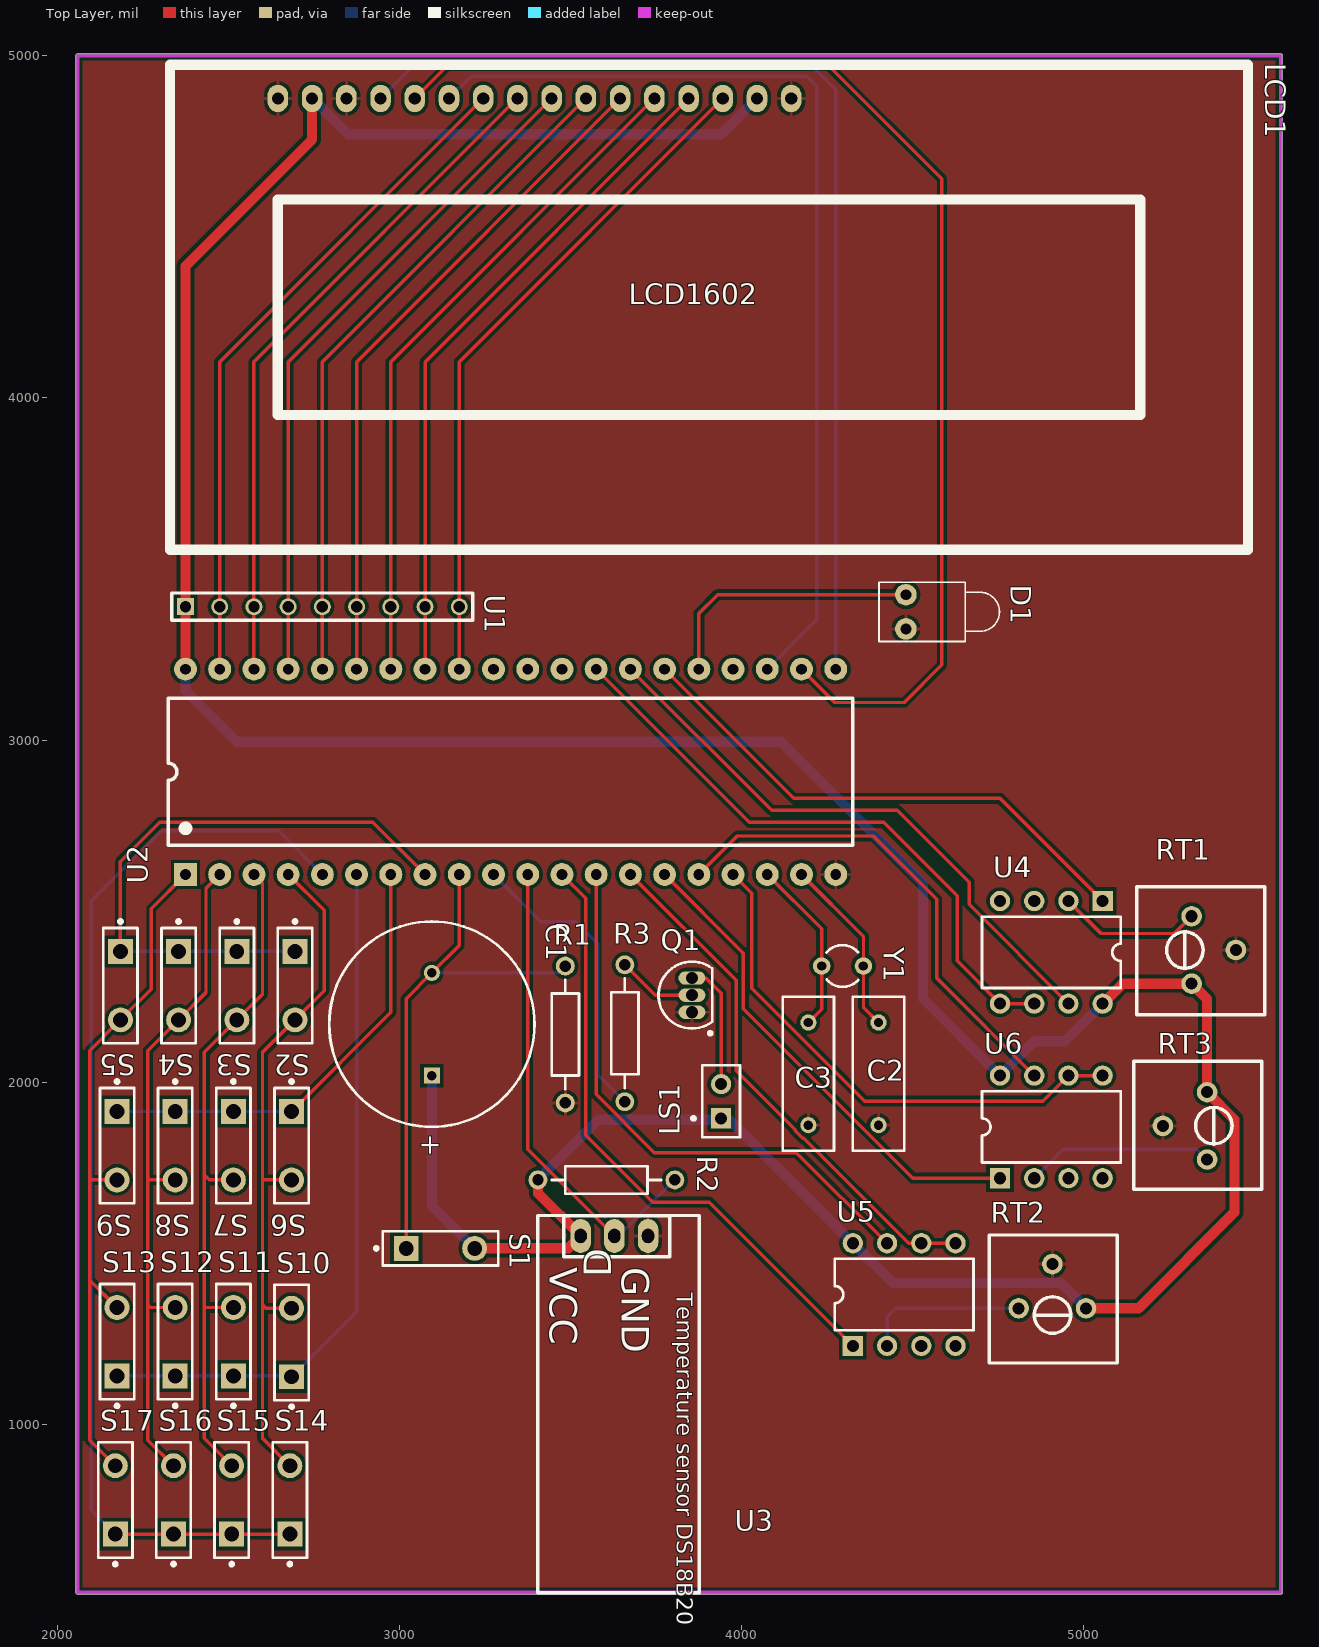
[diagram p0: Top Layer view]
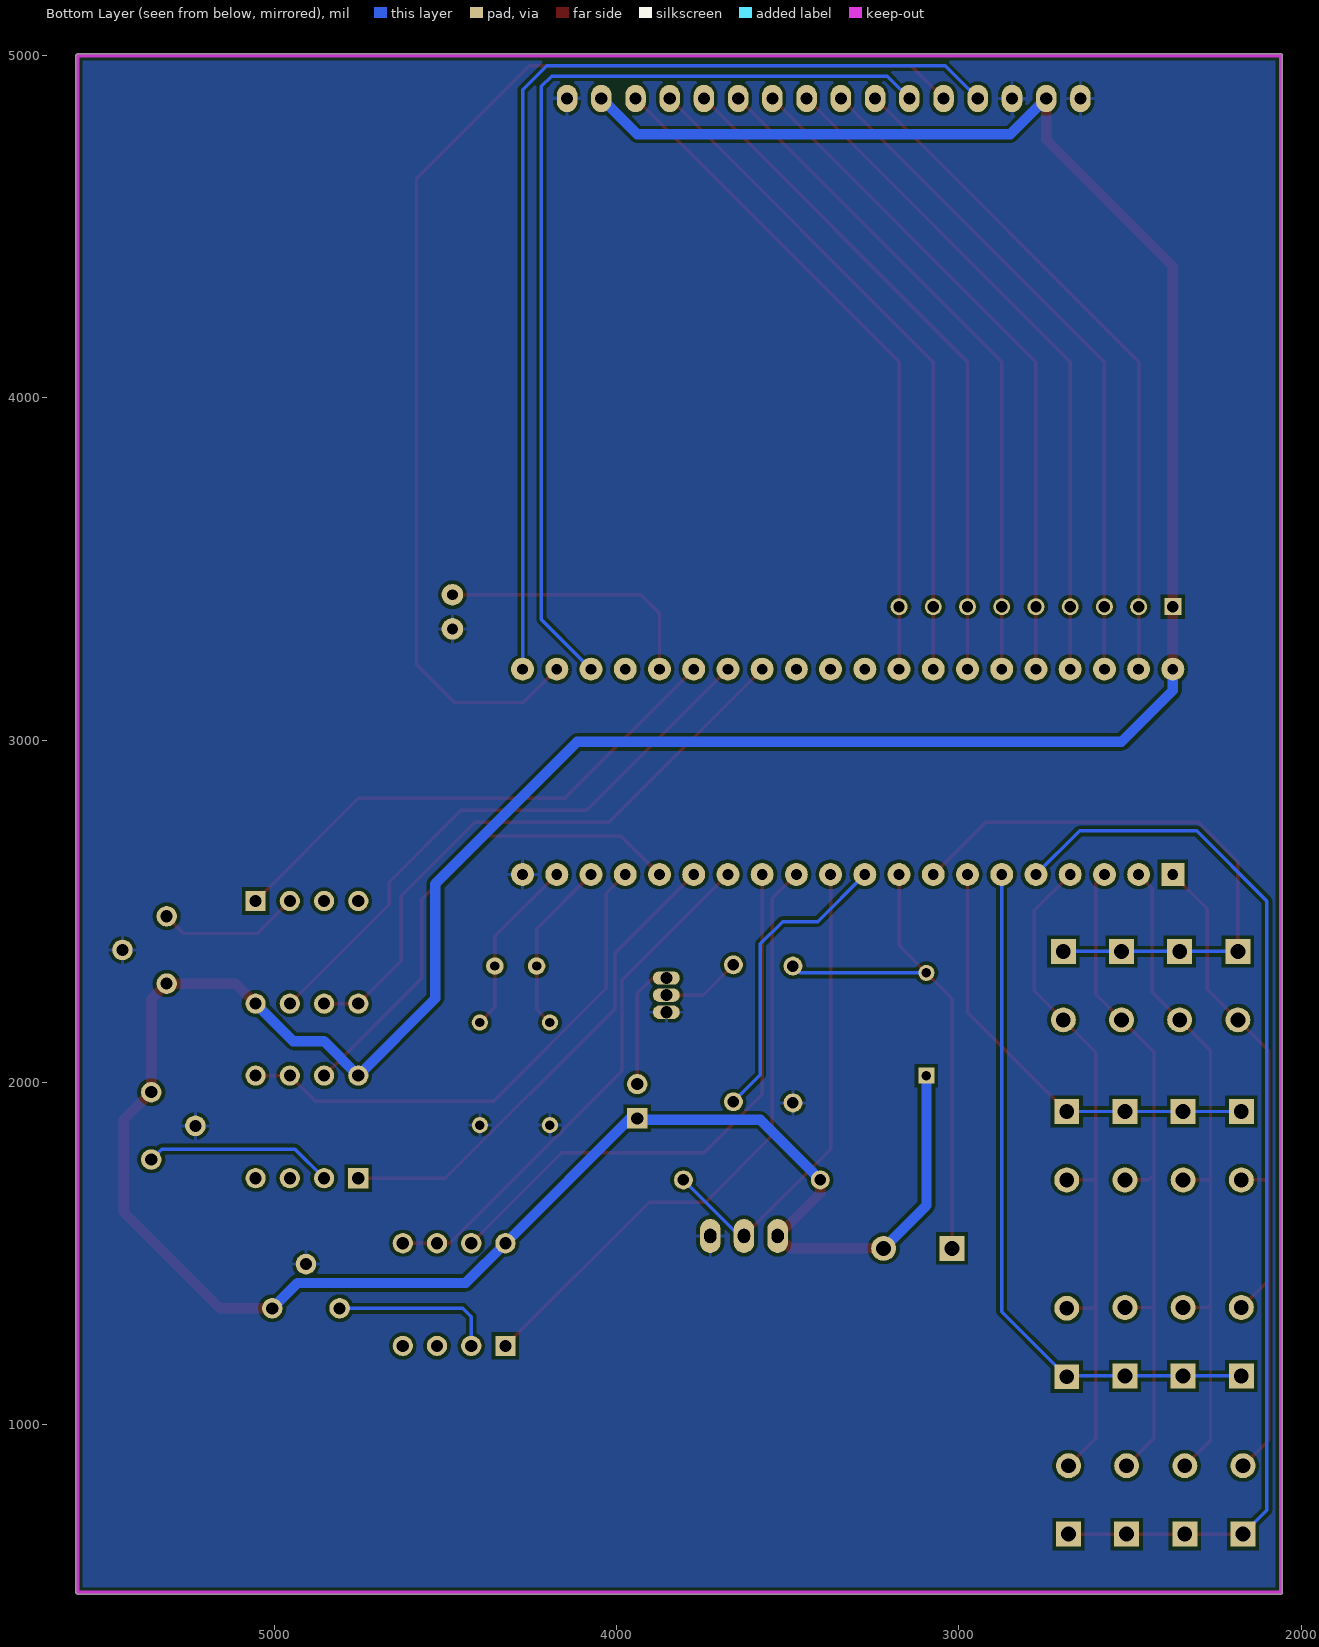
[diagram p1: Bottom Layer view, seen from below]
# Altium PCB MISC80677.PcbDoc
Units mil, origin at the board's own origin, x right, y up, seen from the top; angles counter-clockwise.
Board outline 3525.03 x 4500.03 mil, 2 copper layers (Top Layer, Bottom Layer); 37 components, 42 nets, 156 pads, 0 vias.

## Layer stack, top to bottom (the 12.6 mil dielectric is the usual default, probably not edited)
Top Solder: solder mask 0.4, Solder Resist, Dk 3.5
Top Layer: signal copper 1.4
Dielectric 1: dielectric 12.6, FR-4, Dk 4.8
Bottom Layer: signal copper 1.4
Bottom Solder: solder mask 0.4, Solder Resist, Dk 3.5

## Board outline
2054.99,510 ccw(c2060,510) 2060,504.99 5575,504.99 ccw(c5575,510) 5580.02,510 5580.02,5000 ccw(c5575,5000) 5575,5005.02 2060,5005.02 ccw(c2060,5000) 2054.99,5000

## Design rules (kind name [scope] priority, off if disabled: settings)
Clearance [All] p1: gap=10
MinimumSolderMaskSliver [All] p1: minsoldermaskwidth=0
PolygonConnect [All] p1: connectstyle=Relief reliefconductorwidth=10 reliefentries=4 polygonreliefangle="90 Angle" airgapwidth=10
RoutingVias [All] p1: holewidth=28 width=50 viastyle="Through Hole" minholewidth=28 minwidth=50 maxholewidth=28 maxwidth=50
SilkToSilkClearance [All] p1: silktosilkclearance=0
SilkToSolderMaskClearance [IsPad] p1: minsilkscreentomaskgap=0 clearancetoexposedcopper=TRUE
SolderMaskExpansion [All] p1: expansion=4
Width [All] p1: maxlimit=30 minlimit=10 preferedwidth=10
27 further rules are at their usual default settings.

## Components (designator, comment, footprint, x,y, rotation, side; value= is the part's Value field where it differs from the comment)
C1 "1UF" RB7.6-15 3095,2170 r270 top
C2 "22PF" RAD-0.3 4400,2025 r90 top
C3 "22PF" RAD-0.3 4195,2025 r90 top
D1 "LED1" LED-1 4480,3375 r0 top
LCD1 "LCD1602" LCD1602 2645,4875 r0 top
LS1 "Speaker" PIN2 3940,1895 r90 top
Q1 "2N3904" TO-92A 3855,2255 r0 top
R1 "1K" AXIAL-0.4 3485,2140 r90 top
R2 "1K" AXIAL-0.4 3605,1715 r0 top
R3 "1K" AXIAL-0.4 3658.94,2143.44 r90 top
RT1 "1K" 电位器 5330,2385 r270 top
RT2 "1K" 电位器 4910,1355 r0 top
RT3 "1K" 电位器 5345,1875 r90 top
S1 "SW-PB" SPST-2 3120,1515 r0 top
S2 "SW-PB" SPST-2 2695,2282.72 r270 top
S3 "SW-PB" SPST-2 2525,2282.72 r270 top
S4 "SW-PB" SPST-2 2355,2282.72 r270 top
S5 "SW-PB" SPST-2 2185,2282.72 r270 top
S6 "SW-PB" SPST-2 2685,1815 r270 top
S7 "SW-PB" SPST-2 2515,1815 r270 top
S8 "SW-PB" SPST-2 2345,1815 r270 top
S9 "SW-PB" SPST-2 2175,1815 r270 top
S10 "SW-PB" SPST-2 2685,1240 r90 top
S11 "SW-PB" SPST-2 2515,1242.28 r90 top
S12 "SW-PB" SPST-2 2345,1242.28 r90 top
S13 "SW-PB" SPST-2 2175,1242.28 r90 top
S14 "SW-PB" SPST-2 2680,780 r90 top
S15 "SW-PB" SPST-2 2510,780 r90 top
S16 "SW-PB" SPST-2 2340,780 r90 top
S17 "SW-PB" SPST-2 2170,780 r90 top
U1 "Resistor network" paizu 2775,3390 r0 top
U2 "AT89C52" DIP40 3325,2907.46 r90 top
U3 "DS18B20" DS18B20 3640,1060 r270 top
U4 "ADC0832CCN" N08E 4905,2380 r180 top
U5 "ADC0832CCN" N08E 4475,1380 r0 top
U6 "ADC0832CCN" N08E 4905,1870 r0 top
Y1 "12MHZ" R38 4295,2340 r270 top

## Footprints (in the part's own frame and the unit in brackets; to place one, negate y for a bottom-side part, rotate by r counter-clockwise, add the part's x,y. Pads: shape width x height; smd on the part's side, far side on the other; paste and mask are expansions set on the pad)
AXIAL-0.4 [mm] "Axial Device, Thru-Hole; 2 Leads; 0.4 in Pin Spacing"
  round 1.4 hole 0.85: 1(-5.08,0) 2(5.08,0)
  silkscreen extent -4.06,-1.02 4.06,1.02
DIP40 [mm]
  rect 1.7x1.7 hole 0.8: 1(-7.62,24.13)
  round 1.7 hole 0.8: 2(-7.62,21.59) 3(-7.62,19.05) 4(-7.62,16.51) 5(-7.62,13.97) 6(-7.62,11.43) 7(-7.62,8.89) 8(-7.62,6.35) 9(-7.62,3.81) 10(-7.62,1.27) 11(-7.62,-1.27) 12(-7.62,-3.81) 13(-7.62,-6.35) 14(-7.62,-8.89) 15(-7.62,-11.43) 16(-7.62,-13.97) 17(-7.62,-16.51) 18(-7.62,-19.05) 19(-7.62,-21.59) 20(-7.62,-24.13) 21(7.62,-24.13) 22(7.62,-21.59) 23(7.62,-19.05) 24(7.62,-16.51) 25(7.62,-13.97) 26(7.62,-11.43) 27(7.62,-8.89) 28(7.62,-6.35) 29(7.62,-3.81) 30(7.62,-1.27) 31(7.62,1.27) 32(7.62,3.81) 33(7.62,6.35) 34(7.62,8.89) 35(7.62,11.43) 36(7.62,13.97) 37(7.62,16.51) 38(7.62,19.05) 39(7.62,21.59) 40(7.62,24.13)
  silkscreen extent -5.46,-25.4 5.46,25.4, body extent -7.91,-26.19 7.65,26.16, height 4.7
DS18B20 [mil]
  oval 99.37x60 hole 35.43 slot 41.34 at 0 deg paste+0 mask+4: 1(-491.35,86.55) 2(-491.35,-11.88) 3(-491.35,-110.3)
  silkscreen extent -551,-236 551,236
LCD1602 [mil]
  oval 60x80 hole 35.43: 1(0,0) 2(100,0) 3(200,0) 4(300,0) 5(400,0) 6(500,0) 7(600,0) 8(700,0) 9(800,0) 10(900,0) 11(1000,0) 12(1100,0) 13(1200,0) 14(1300,0) 15(1400,0) 16(1500,0)
  silkscreen extent -315,-1319 2835,98, body extent -315,-1357 2854,80, height 414
LED-1 [mm] "LED; 2 Leads"
  round 1.6 hole 0.8: 1(0,1.27) 2(0,-1.27)
  silkscreen extent -2,-2.2 6.95,2.2
N08E [mm] "DIP; 8 Leads; Row Spacing 7.62 mm; Pitch 2.54 mm"
  rect 1.5x1.5 hole 0.9: 1(-3.81,-3.81)
  round 1.5 hole 0.9: 2(-1.27,-3.81) 3(1.27,-3.81) 4(3.81,-3.81) 5(3.81,3.81) 6(1.27,3.81) 7(-1.27,3.81) 8(-3.81,3.81)
  silkscreen extent -5.15,-2.65 5.15,2.65
paizu [mm]
  rect 1.26x1.26 hole 0.84 paste+0 mask+0.051: 1(-10.16,0)
  round 1.26 hole 0.84 paste+0 mask+0.051: 2(-7.62,0) 3(-5.08,0) 4(-2.54,0) 5(0,0) 6(2.54,0) 7(5.08,0) 8(7.62,0) 9(10.16,0)
  silkscreen extent -11.18,-1.02 11.18,1.02
PIN2 [mm] "Photosensitive Diode; 2 Leads"
  rect 1.5x1.5 hole 0.9: 1(0,0)
  round 1.5 hole 0.9: 2(2.54,0)
  silkscreen extent -1.4,-1.4 3.94,2.17
R38 [mm] "Crystal, Thru-Hole; 2 Leads; Body 3.1 x 8.2 mm (Dia.xH)"
  round 1.3 hole 0.7: 1(0,1.55) 2(0,-1.55)
  silkscreen extent -1.55,-1.19 1.55,1.17
RAD-0.3 [mm] "Radial Cap, Thru-Hole; 2 Leads; 0.3 in Pin Spacing"
  round 1.2 hole 0.7: 1(-3.81,0) 2(3.81,0)
  silkscreen extent -5.71,-1.91 5.71,1.91
RB7.6-15 [mm] "Polarized Capacitor (Radial); 2 Leads"
  rect 1.2x1.2 hole 0.7: 1(3.81,0)
  round 1.2 hole 0.7: 2(-3.81,0)
  silkscreen extent -7.62,-7.62 7.62,7.62
SPST-2 [mm] "Switch; 2 Leads"
  rect 1.85x1.85 hole 1.1: 1(-2.54,0)
  round 1.85 hole 1.1: 2(2.54,0)
  silkscreen extent -4.89,-1.27 4.28,1.27
TO-92A [mm] "TO, Flat Index; 3 In-Line, Axial Leads; Body Dia. 4.5mm; Leads 0.51 x 0.48 mm (max)"
  oval 2x1 hole 0.9: 1(0,-1.27) 2(0,0) 3(0,1.27)
  silkscreen extent -2.48,-2.95 1.5,2.48, body extent -2.48,-2.5 1.5,2.5, height 6.86
电位器 [mil]
  round 60 hole 35.43 paste+0 mask+2: 1(96.41,-15.12) 2(-2.01,114.1) 3(-100.44,-15.12)
  silkscreen extent -187,-175 187,199

## Part data
C1: library part "Cap Pol1", "Polarized Capacitor (Radial)"
C2 C3: library part Cap, "Capacitor"
D1: "Typical RED GaAs LED"
LS1: "Loudspeaker"
Q1: "NPN General Purpose Amplifier"
R1 R2 R3: library part Res2, "Resistor"
RT1 RT2 RT3: library part 电位器
S1 S2 S3 S4 S5 S6 S7 S8 S9 S10 S11 S12 S13 S14 S15 S16 S17: "Switch"
U1: library part 排阻
U2: library part STC89C52
U4 U5 U6: "8-Bit Serial I/O A/D Converter with Multiplexer Option"
Y1: library part XTAL, "Crystal Oscillator"

## Nets (pads, with @x,y where several pads share a name; then routed paths per layer and width w, separated by ;. In a path a pad name is that pad's centre, name@x,y a point inside that pad or via, vN(x,y) a via of type N, cw(c..) or ccw(c..) an arc to the next point about the centre after c; other vN are vias at no path point)
D0: LCD1.7 U1.2 U2.39 | length 1986.5
  Top Layer w10: U2.39 U1.2 2475,4105 LCD1.7
D1: LCD1.8 U1.3 U2.38 | length 1986.5
  Top Layer w10: U2.38 U1.3 2575,4105 LCD1.8
D2: LCD1.9 U1.4 U2.37 | length 1986.5
  Top Layer w10: U2.37 U1.4 2675,4105 LCD1.9
D3: LCD1.10 U1.5 U2.36 | length 1986.5
  Top Layer w10: U2.36 U1.5 2775,4105 LCD1.10
D4: LCD1.11 U1.6 U2.35 | length 1986.5
  Top Layer w10: U2.35 U1.6 2875,4105 LCD1.11
D5: LCD1.12 U1.7 U2.34 | length 1986.5
  Top Layer w10: U2.34 U1.7 2975,4105 LCD1.12
D6: LCD1.13 U1.8 U2.33 | length 1986.5
  Top Layer w10: U2.33 U1.8 3075,4105 LCD1.13
D7: LCD1.14 U1.9 U2.32 | length 1986.5
  Top Layer w10: U2.32 U1.9 3175,4105 LCD1.14
GND: C2.1 C3.1 D1.2 LCD1.1 LCD1.3 LCD1.16 Q1.1 R1.1 RT1.2 RT2.2 RT3.2 U2.20 U3.1
NetC2_2: C2.2 U2.19 Y1.1 | length 525.7
  Top Layer w10: U2.19 4356.02,2426.44 Y1.1 4356.02,2218.98 C2.2
NetC3_2: C3.2 U2.18 Y1.2 | length 514.5
  Top Layer w10: U2.18 4233.98,2448.49 Y1.2 4233.98,2213.98 C3.2
NetLS1_2: LS1.2 Q1.3 | length 368.6
  Top Layer w10: Q1.3 3895,2305 3940,2260 LS1.2
NetQ1_2: Q1.2 R3.2 | length 232.7
  Top Layer w10: R3.2 3747.38,2255 Q1.2
NetRT1_3: RT1.3 U4.2 | length 420.1
  Top Layer w10: U4.2 5050,2435 5264.44,2435 RT1.3
NetRT2_3: RT2.3 U5.2 | length 479.9
  Bottom Layer w10: U5.2 4425,1315 4449.88,1339.88 RT2.3
NetRT3_3: RT3.3 U6.2 | length 552.9
  Bottom Layer w10: U6.2 4940,1805 5329.68,1805 RT3.3
P1.0: S5.2 S9.2 S13.2 S17.2 U2.1 | length 2067.6
  Top Layer w10: S17.2 2095,955 2095,1422.28 ; S13.2 2095,1422.28 ; S9.2 2095,1715 ; U2.1 2275,2507.46 2275,2272.72 S5.2 2095,2092.72 2095,1715 ; 2095,1422.28 2095,1715
P1.1: S4.2 S8.2 S12.2 S16.2 U2.2 | length 2011.3
  Top Layer w10: S16.2 2265,955 2265,1350 ; S12.2 2272.72,1342.28 2265,1350 ; S8.2 2271.36,1715 2265,1721.36 ; U2.2 2435,2567.46 2435,2262.72 S4.2 2265,2092.72 2265,1721.36 ; 2265,1350 2265,1721.36
P1.2: S3.2 S7.2 S11.2 S15.2 U2.3 | length 2018.7
  Top Layer w10: S15.2 2430,960 2430,1345 ; S11.2 2432.72,1342.28 2430,1345 ; S7.2 2445,1715 2430,1730 ; U2.3 2600,2582.46 2600,2257.72 S3.2 2430,2087.72 2430,1730 ; 2430,1345 2430,1730
P1.3: S2.2 S6.2 S10.2 S14.2 U2.4 | length 2054.9
  Top Layer w10: U2.4 2780,2502.46 2780,2267.72 S2.2 2600,2087.72 2600,1720 ; S14.2 2600,960 2600,1350 ; S10.2 2610,1340 2600,1350 ; S6.2 2605,1715 2600,1720 ; 2600,1350 2600,1720
P1.4: S14.1 S15.1 S16.1 S17.1 U2.5 | length 3201.7
  Top Layer w10: S17.1 S16.1 S15.1 S14.1
  Bottom Layer w10: S17.1 2100,750 2100,2530 2305,2735 2647.46,2735 U2.5
P1.5: S10.1 S11.1 S12.1 S13.1 U2.6 | length 2057.1
  Bottom Layer w10: S13.1 S12.1 S11.1 2682.72,1142.28 S10.1 2875,1330 U2.6
P1.6: S6.1 S7.1 S8.1 S9.1 U2.7 | length 1322.6
  Top Layer w10: S6.1 2975,2205 U2.7
  Bottom Layer w10: S9.1 S8.1 S7.1 S6.1
P1.7: S2.1 S3.1 S4.1 S5.1 U2.8 | length 1773.1
  Top Layer w10: S5.1 2185,2645 2300,2760 2922.46,2760 U2.8
  Bottom Layer w10: S5.1 S4.1 S3.1 S2.1
P2.0: LCD1.4 U2.21 | length 3090.9
  Bottom Layer w10: LCD1.4 3040,4970 4205,4970 4275,4900 U2.21
P2.1: LCD1.5 U2.22 | length 3632
  Top Layer w10: LCD1.5 3140,4970 4255,4970 4585,4640 4585,3220 4475,3110 4272.46,3110 U2.22
P2.2: LCD1.6 U2.23 | length 2876.9
  Bottom Layer w10: LCD1.6 3210,4940 4190,4940 4220,4910 4220,3352.46 U2.23
P2.3: U2.24
P2.4: D1.1 U2.25 | length 790.3
  Top Layer w10: U2.25 3875,3370 3930,3425 D1.1
P2.5: U2.26 U4.1 | length 1560.6
  Top Layer w10: U2.26 4152.46,2830 4755,2830 U4.1
P2.6: U2.27 U4.7 | length 1723
  Top Layer w10: U2.27 4087.46,2795 4455,2795 4665,2585 4665,2520 U4.7
P2.7: U2.28 U4.5 U4.6 | length 1796.2
  Top Layer w10: U2.28 4022.46,2760 4415,2760 4630,2545 4630,2355 U4.5 U4.6
P3.0: R3.1 U2.10 | length 883.1
  Bottom Layer w10: U2.10 3412.46,2470 3515,2470 3580,2405 3580,2022.38 R3.1
P3.1: R2.2 U2.11 U3.2 | length 1405.6
  Top Layer w10: U2.11 3375,1805.19 3628.12,1552.07 U3.2
  Bottom Layer w10: U3.2 3641.35,1551.35 R2.2
P3.2: U2.12 U5.1 | length 1826.2
  Top Layer w10: U2.12 3545,2537.46 3545,1845 3740,1650 3905,1650 U5.1
P3.3: U2.13 U5.7 | length 1672.6
  Top Layer w10: U2.13 3575,1965 3745,1795 4160,1795 U5.7
P3.4: U2.14 U5.5 U5.6 | length 1552.8
  Top Layer w10: U2.14 3984.53,2297.94 3984.53,2033.44 4156.38,1861.59 4156.38,1859 4179,1836.38 4181.59,1836.38 4487.97,1530 U5.6 U5.5
P3.5: U2.15 U6.1 | length 1442.5
  Top Layer w10: U2.15 4005,2377.46 4005,2215.38 4500.38,1720 U6.1
P3.6: U2.16 U6.7 | length 1451.3
  Top Layer w10: U2.16 3987.54,2720 4385,2720 4570,2535 4570,2305 U6.7
P3.7: U2.17 U6.5 U6.6 | length 1548
  Top Layer w10: U2.17 4030,2552.46 4030,2275 4360,1945 4880,1945 U6.6 U6.5
RST: C1.2 R1.2 S1.1 U2.9 | length 1555
  Top Layer w10: S1.1 3020,2245 C1.2 3175,2400 U2.9
  Bottom Layer w10: C1.2 3465,2320 R1.2
VCC: C1.1 LCD1.2 LCD1.15 LS1.1 R2.1 RT1.1 RT2.1 RT3.1 S1.2 U1.1 U2.40 U3.3 U4.8 U5.8 U6.8 | length 11256.4
  Top Layer w30: U2.40 U1.1 2375,4385 2745,4755 LCD1.2 ; S1.2 3493.35,1515 U3.3 3405,1676.05 R2.1 ; RT2.1 5159.88,1339.88 5440,1620 5440,1891.53 RT3.1 5360.12,2243.36 RT1.1 5113.59,2288.59 U4.8
  Bottom Layer w30: U2.40 2375,3145 2525,2995 4115,2995 4530,2580 4530,2245 U6.8 4855,2120 4945,2120 U4.8 ; LCD1.2 2850,4770 3940,4770 LCD1.15 ; C1.1 3095,1640 S1.2 ; R2.1 3580.88,1890.88 3935.88,1890.88 LS1.1 3960,1895 U5.8 4440.9,1414.1 4932.19,1414.1 RT2.1
pads on no net: U2.29 U2.30 U2.31 U4.3 U4.4 U5.3 U5.4 U6.3 U6.4

## Polygon pours and split planes (outlines as drawn)
GND on Bottom Layer "G" (solid, remove dead copper, pour order 0): 975,5205 6140,5205 6205,5270 6020,5085 6020,195 1175,195 815,555
GND on Top Layer "G" (solid, remove dead copper, pour order 2): 1300,5250 1310,5260 6075,5260 6075,235 5840,0 5655,185 315,185

## Keep-outs
Keep-Out Layer:
  lines w10: 2200,5000 5575,5000 5575,2025 5575,640 5575,510 5560,510 ; 2230,5000 2060,5000 2060,510 3675,510 ; 3655,510 5570,510